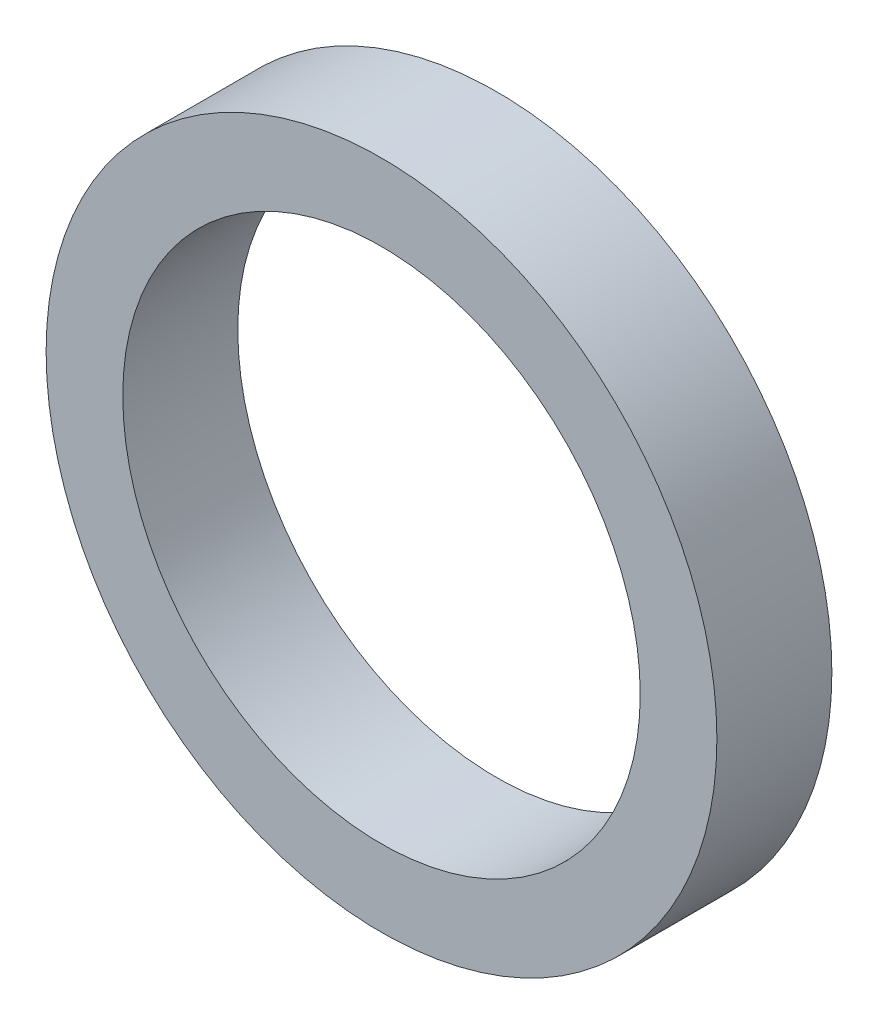
SolidWorks part; units mm, degrees
ref_plane "Front Plane" through (0, 0, 0) normal (0, 0, 1) x (1, 0, 0)
ref_plane "Top Plane" through (0, 0, 0) normal (0, 1, 0) x (1, 0, 0)
ref_plane "Right Plane" through (0, 0, 0) normal (1, 0, 0) x (0, 0, -1)
sketch "Sketch1" plane through (0, 0, 0) normal (0, 0, 1) x (1, 0, 0)
  circle A0 centre (0, 0) radius 17.5
  circle A1 centre (0, 0) radius 13.5
  dimension "D1" = 35
  dimension "D2" = 27
extrude "Boss-Extrude1" add sketch "Sketch1" along normal blind 6
